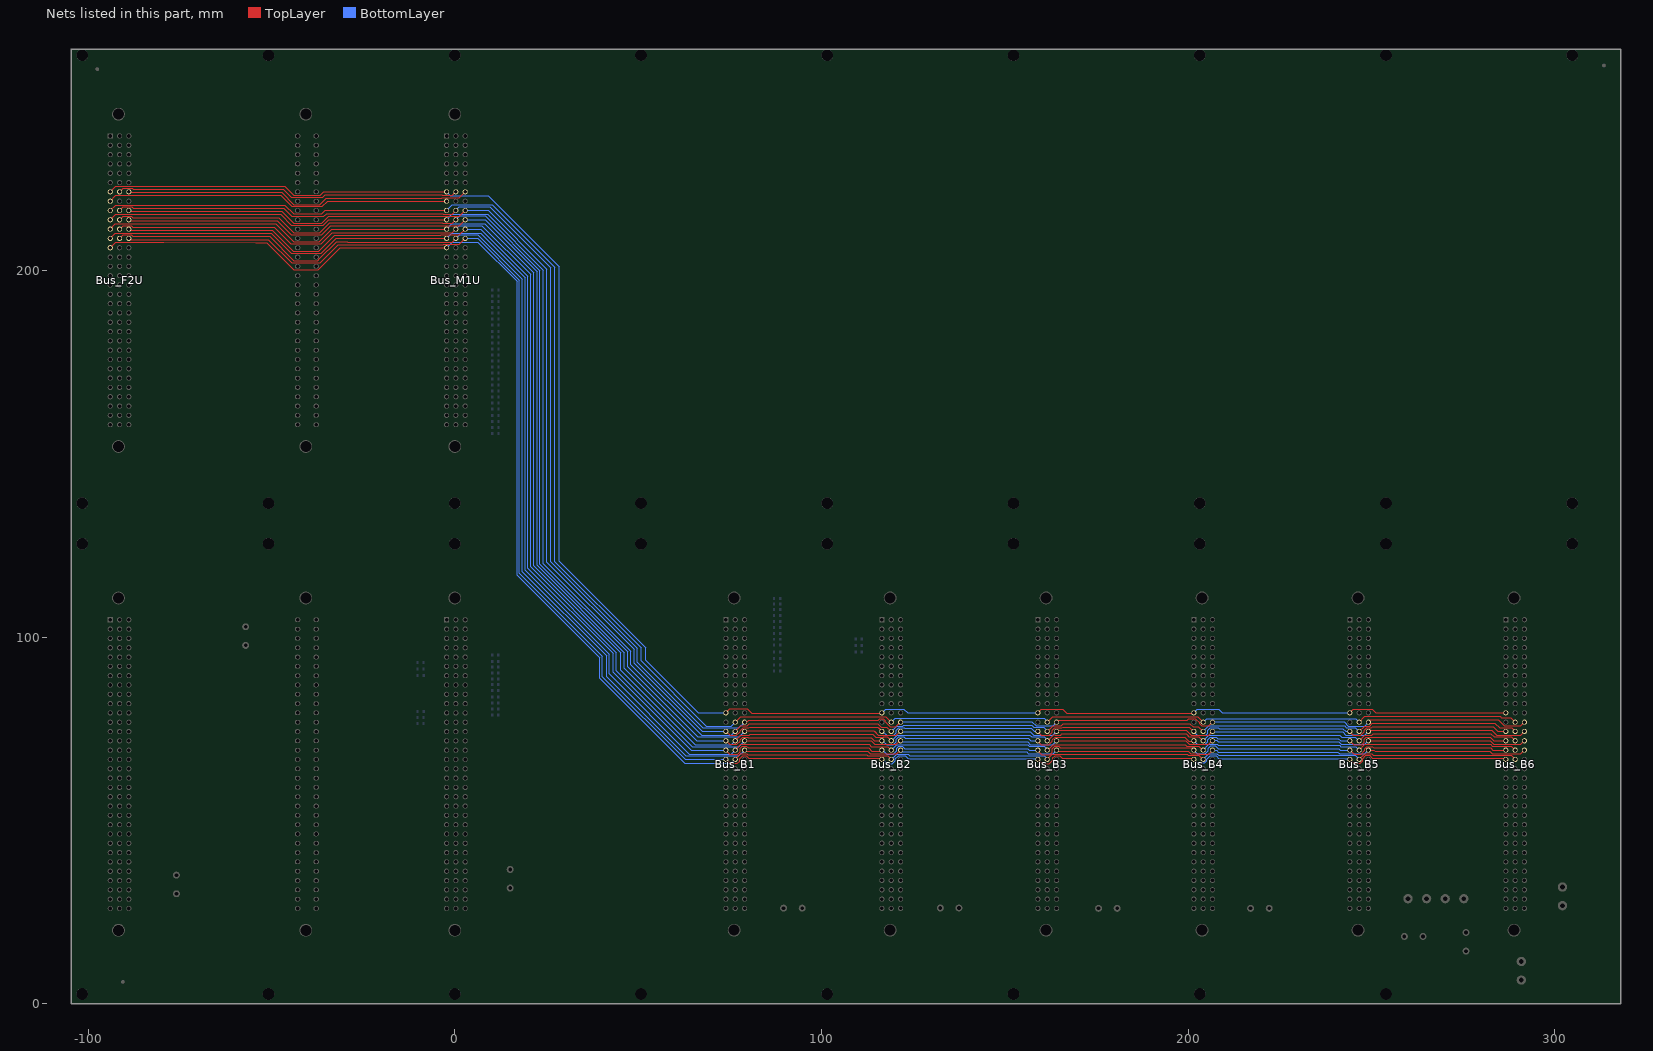
[diagram p0: the nets of this part, all layers, seen from the top]
# Altium PCB MISC67337.PcbDoc (part 5 of 7)
Units mm, origin at the board's own origin, x right, y up, seen from the top; angles counter-clockwise.
Board outline 422.71 x 260.35 mm, 4 copper layers (TopLayer, InternalPlane1, InternalPlane2, BottomLayer); 82 components, 143 nets, 1295 pads, 42 vias.

## Via types
v1: diameter 0.61, hole 0.305, TopLayer to BottomLayer, 42 vias

## Nets (pads, with @x,y where several pads share a name; then routed paths per layer and width w, separated by ;. In a path a pad name is that pad's centre, name@x,y a point inside that pad or via, vN(x,y) a via of type N, cw(c..) or ccw(c..) an arc to the next point about the centre after c; other vN are vias at no path point) (continued)
B_DSP2_XA12: Bus_B1.A11 Bus_B2.A11 Bus_B3.A11 Bus_B4.A11 Bus_B5.A11 Bus_B6.A11 Bus_F2U.A7 Bus_M1U.A7 | length 496.5
  TopLayer w0.254: Bus_F2U.A7@-93.97,221.413 -92.407,222.976 ; -92.407,222.965 -46.384,222.965 -43.891,220.472 -36.703,220.472 -35.762,221.413 -34.544,221.413 ; -35.285,221.413 -34.544,221.413 ; Bus_M1U.A7@-2.373,221.28 Bus_M1U.A7@-2.24,221.413 ; Bus_M1U.A7@-2.373,221.413 -34.544,221.413 ; Bus_B1.A11@73.96,79.44 74.938,80.418 79.754,80.418 80.964,79.208 81.661,79.208 ; 81.117,79.208 81.661,79.208 ; Bus_B2.A11@116.316,79.208 81.661,79.208 ; Bus_B2.A11@116.316,79.502 Bus_B2.A11@116.505,79.313 ; Bus_B3.A11@159.05,79.313 160.028,80.291 165.835,80.291 166.879,79.247 Bus_B4.A11@201.406,79.247 ; Bus_B4.A11@201.406,79.375 Bus_B4.A11@201.595,79.186 ; Bus_B5.A11@244.14,79.313 245.118,80.291 250.214,80.291 251.193,79.312 Bus_B6.A11@286.685,79.312
  BottomLayer w0.254: Bus_M1U.A7@-2.24,221.413 -1.172,220.345 9.144,220.345 28.448,201.041 28.448,120.65 52.07,97.028 52.07,93.599 66.356,79.313 Bus_B1.A11@73.955,79.313 ; Bus_B2.A11@116.632,79.375 117.61,80.353 122.453,80.353 123.493,79.313 Bus_B3.A11@159.05,79.313 ; Bus_B3.A11@159.144,79.408 Bus_B3.A11@159.177,79.375 ; Bus_B4.A11@201.595,79.313 202.548,80.266 203.706,80.266 ; 203.73,80.291 207.188,80.291 ; 207.467,80.291 207.188,80.291 ; Bus_B5.A11@244.14,79.313 209.383,79.313 208.405,80.291 207.188,80.291
B_DSP2_XA13: Bus_F2U.B7 Bus_M1U.B7 | length 98.4
  TopLayer w0.254: Bus_F2U.B7@-91.43,221.413 -90.452,222.391 -88.001,222.391 -87.732,222.122 -49.581,222.122 ; -47.255,222.122 -49.581,222.122 ; -35.012,220.567 -32.817,220.567 ; Bus_M1U.B7@0.3,221.413 -0.678,220.436 -3.469,220.436 -3.6,220.567 -32.817,220.567 ; -49.581,222.122 -46.76,222.122 -44.602,219.964 -35.992,219.964 -35.389,220.567 -32.817,220.567
B_DSP2_XA14: Bus_F2U.C7 Bus_M1U.C7 | length 94.5
  TopLayer w0.254: Bus_F2U.C7@-88.89,221.279 -47.187,221.279 -43.867,217.959 -36.803,217.959 -35.042,219.72 -3.521,219.72 -3.389,219.851 1.278,219.851 Bus_M1U.C7@2.84,221.413
B_DSP2_XA15: Bus_F2U.A8 Bus_M1U.A8 | length 94.2
  TopLayer w0.254: Bus_F2U.A8@-93.97,218.873 -92.407,220.436 -47.487,220.436 -44.475,217.424 -36.119,217.424 -34.669,218.873 Bus_M1U.A8@-2.24,218.873
B_DSP2_XD0: Bus_B1.B12 Bus_B2.B12 Bus_B3.B12 Bus_B4.B12 Bus_B5.B12 Bus_B6.B12 Bus_F2U.A9 Bus_M1U.A9 | length 503.7
  TopLayer w0.254: Bus_F2U.A9@-93.97,216.333 -92.498,217.805 -46.355,217.805 -43.942,215.392 -36.271,215.392 -35.33,216.333 Bus_M1U.A9@-2.24,216.333 ; Bus_B1.B12@76.495,76.773 77.984,78.262 117.556,78.262 Bus_B2.B12@119.045,76.773 ; 162.974,78.157 Bus_B3.B12@161.59,76.773 163.115,78.298 202.61,78.298 Bus_B4.B12@204.135,76.773 202.751,78.157 ; Bus_B5.B12@246.68,76.773 248.242,78.335 249.625,78.335 249.65,78.36 285.14,78.36 285.471,78.029 287.969,78.029 Bus_B6.B12@289.225,76.773
  BottomLayer w0.254: Bus_M1U.A9@-2.24,216.333 -0.678,217.896 10.247,217.896 27.305,200.838 27.305,120.523 50.8,97.028 50.8,93.472 68.58,75.692 75.414,75.692 Bus_B1.B12@76.495,76.773 ; Bus_B2.B12@119.172,76.835 120.15,77.813 160.739,77.813 Bus_B3.B12@161.717,76.835 ; Bus_B4.B12@204.135,76.773 205.113,77.751 245.702,77.751 Bus_B5.B12@246.68,76.773
B_DSP2_XD1: Bus_B1.C12 Bus_B2.C12 Bus_B3.C12 Bus_B4.C12 Bus_B5.C12 Bus_B6.C12 Bus_F2U.B9 Bus_M1U.B9 | length 504.6
  TopLayer w0.254: Bus_F2U.B9@-91.43,216.333 -90.452,217.311 -88.093,217.311 -87.732,216.95 -46.592,216.95 -44.399,214.757 -35.712,214.757 -34.983,215.487 -3.219,215.487 -3.088,215.356 -0.678,215.356 Bus_M1U.B9@0.3,216.333 ; Bus_B1.C12@79.035,76.773 79.67,76.773 80.213,77.316 112.547,77.316 ; 114.111,77.316 112.547,77.316 ; Bus_B2.C12@121.585,76.9 120.25,75.565 118.745,75.565 117.483,76.827 117.483,77.178 116.91,77.751 115.978,77.751 115.543,77.316 112.547,77.316 ; Bus_B3.C12@164.13,76.808 164.165,76.808 164.707,77.35 197.587,77.35 ; 199.201,77.35 197.587,77.35 ; Bus_B4.C12@206.675,76.773 205.697,75.795 203.73,75.795 203.157,76.368 203.157,76.594 202,77.751 200.179,77.751 199.778,77.35 197.587,77.35 ; Bus_B5.C12@249.22,76.773 249.854,77.407 284.644,77.407 286.256,75.795 290.787,75.795 Bus_B6.C12@291.765,76.773
  BottomLayer w0.254: Bus_M1U.B9@0.3,216.333 1.278,217.311 9.536,217.311 26.162,200.685 26.162,120.523 49.784,96.901 49.784,93.091 67.664,75.211 77.473,75.211 Bus_B1.C12@79.035,76.773 ; Bus_B2.C12@121.712,76.897 157.418,76.897 158.536,75.779 163.201,75.779 Bus_B3.C12@164.257,76.835 ; Bus_B4.C12@206.675,76.839 242.591,76.839 243.713,75.717 248.164,75.717 Bus_B5.C12@249.22,76.773
B_DSP2_XD2: Bus_B1.A13 Bus_B2.A13 Bus_B3.A13 Bus_B4.A13 Bus_B5.A13 Bus_B6.A13 Bus_F2U.C9 Bus_M1U.C9 | length 502.2
  TopLayer w0.254: Bus_F2U.C9@-88.89,216.095 -48.514,216.095 ; -47.804,216.095 -48.514,216.095 ; Bus_M1U.C9@2.84,216.333 1.278,214.771 -34.403,214.771 -36.295,212.879 -43.921,212.879 -47.137,216.095 -48.514,216.095 ; Bus_B1.A13@73.96,74.36 75.168,73.152 76.835,73.152 77.851,74.168 77.851,74.432 78.63,75.211 80.188,75.211 80.401,75.424 115.314,75.424 Bus_B2.A13@116.505,74.233 ; 115.654,75.211 Bus_B2.A13@116.505,74.36 ; Bus_B3.A13@159.05,74.233 160.028,73.255 162.155,73.255 162.941,74.041 162.941,74.549 163.603,75.211 165.583,75.211 165.825,75.453 200.375,75.453 Bus_B4.A13@201.595,74.233 200.517,75.311 ; Bus_B5.A13@244.14,74.233 245.118,73.255 247.118,73.255 248.031,74.168 248.031,74.549 248.693,75.211 250.038,75.211 250.329,75.502 283.273,75.502 284.542,74.233 Bus_B6.A13@286.685,74.233
  BottomLayer w0.254: Bus_M1U.C9@2.84,216.333 9.168,216.333 25.146,200.355 25.146,120.396 48.895,96.647 48.895,92.837 67.499,74.233 Bus_B1.A13@73.955,74.233 ; Bus_B2.A13@116.632,74.295 117.775,73.152 119.699,73.152 120.396,73.849 120.396,74.611 121.071,75.286 122.407,75.286 122.582,75.286 122.803,75.065 155.956,75.065 ; 156.972,75.065 155.956,75.065 ; Bus_B3.A13@159.177,74.295 158.05,74.295 157.28,75.065 155.956,75.065 ; Bus_B4.A13@201.595,74.233 202.573,73.255 204.827,73.255 205.359,73.787 205.359,74.549 206.032,75.222 ; 206.121,75.222 206.032,75.222 ; 241.935,75.015 241.198,75.015 ; Bus_B5.A13@244.14,74.233 243.013,74.233 242.231,75.015 241.198,75.015 ; 206.032,75.222 206.07,75.26 208.289,75.26 208.534,75.015 241.198,75.015
B_DSP2_XD3: Bus_B1.B13 Bus_B2.B13 Bus_B3.B13 Bus_B4.B13 Bus_B5.B13 Bus_B6.B13 Bus_F2U.A10 Bus_M1U.A10 | length 506.3
  TopLayer w0.254: Bus_F2U.A10@-93.97,213.793 -92.523,215.24 -47.498,215.24 -44.602,212.344 -35.814,212.344 -34.365,213.793 Bus_M1U.A10@-2.315,213.793 ; Bus_M1U.A10@-2.315,213.868 Bus_M1U.A10@-2.24,213.793 ; Bus_B1.B13@76.495,74.233 78.057,75.795 79.807,75.795 80.382,76.37 115.4,76.37 116.332,75.438 ; Bus_B1.B13@76.5,74.233 77.46,75.194 ; 116.068,75.702 116.332,75.438 ; Bus_B2.B13@119.045,74.233 117.84,75.438 116.332,75.438 ; Bus_B3.B13@161.653,74.17 163.302,75.818 ; 163.424,75.818 163.447,75.795 165.408,75.795 166.014,76.402 200.509,76.402 201.379,75.532 202.836,75.532 Bus_B4.B13@204.135,74.233 ; Bus_B4.B13@204.071,74.17 Bus_B4.B13@204.135,74.106 ; Bus_B5.B13@246.68,74.233 248.139,75.692 249.522,75.692 250.285,76.455 252.603,76.455 ; 250.698,76.455 252.603,76.455 ; Bus_B6.B13@289.225,74.233 288.247,75.211 284.961,75.211 283.717,76.455 252.603,76.455
  BottomLayer w0.254: Bus_M1U.A10@-2.24,213.793 -0.768,215.265 8.966,215.265 24.13,200.101 24.13,120.015 48.006,96.139 48.006,92.456 67.31,73.152 75.414,73.152 Bus_B1.B13@76.495,74.233 ; Bus_B2.B13@119.172,74.295 120.569,75.692 122.239,75.692 122.528,75.981 157.318,75.981 157.926,75.373 160.639,75.373 Bus_B3.B13@161.717,74.295 ; Bus_B4.B13@204.135,74.233 205.697,75.795 242.721,75.795 243.205,75.311 245.602,75.311 Bus_B5.B13@246.68,74.233
B_DSP2_XD4: Bus_B1.C13 Bus_B2.C13 Bus_B3.C13 Bus_B4.C13 Bus_B5.C13 Bus_B6.C13 Bus_F2U.B10 Bus_M1U.B10 | length 502.2
  TopLayer w0.254: Bus_F2U.B10@-91.43,213.793 -90.441,214.782 -88.18,214.782 -87.782,214.384 ; -87.808,214.384 -87.782,214.384 ; Bus_M1U.B10@0.3,213.793 -0.678,212.816 -3.291,212.816 -3.422,212.947 -34.144,212.947 -36.779,210.312 -43.891,210.312 -47.964,214.384 -87.782,214.384 ; Bus_B1.C13@79.04,74.478 114.244,74.478 115.456,73.266 ; 114.489,74.233 115.456,73.266 ; Bus_B2.C13@121.585,74.36 120.377,73.152 115.57,73.152 115.456,73.266 ; Bus_B3.C13@164.13,74.505 199.563,74.505 200.812,73.255 205.697,73.255 Bus_B4.C13@206.675,74.233 ; Bus_B5.C13@249.22,74.233 Bus_B5.C13@249.282,74.295 ; Bus_B5.C13@249.282,74.55 282.904,74.55 284.199,73.255 290.787,73.255 Bus_B6.C13@291.765,74.233
  BottomLayer w0.254: Bus_M1U.B10@0.3,213.793 1.365,214.859 8.306,214.859 23.241,199.923 23.241,119.888 47.117,96.012 47.117,91.948 66.319,72.746 77.548,72.746 Bus_B1.C13@79.035,74.233 ; Bus_B2.C13@121.712,74.149 156.926,74.149 157.923,73.152 163.114,73.152 Bus_B3.C13@164.257,74.295 ; Bus_B4.C13@206.675,74.103 209.499,74.103 242.203,74.103 243.051,73.255 244.832,73.255 244.856,73.279 246.251,73.279 246.275,73.255 248.242,73.255 Bus_B5.C13@249.22,74.233
B_DSP2_XD5: Bus_B1.A14 Bus_B2.A14 Bus_B3.A14 Bus_B4.A14 Bus_B5.A14 Bus_B6.A14 Bus_F2U.C10 Bus_M1U.C10 | length 501.1
  TopLayer w0.254: Bus_F2U.C10@-88.89,213.529 -50.267,213.529 ; -49.074,213.529 -50.267,213.529 ; Bus_M1U.C10@2.84,213.793 1.278,212.231 -33.768,212.231 -36.322,209.677 -44.552,209.677 -48.404,213.529 -50.267,213.529 ; Bus_B1.A14@73.96,71.693 74.938,70.715 76.938,70.715 77.851,71.628 77.851,72.009 78.513,72.671 79.907,72.671 79.991,72.587 113.545,72.587 114.402,71.73 116.468,71.73 Bus_B2.A14@116.505,71.693 ; Bus_B3.A14@159.05,71.566 160.028,70.588 162.028,70.588 162.941,71.501 162.941,71.882 163.152,72.093 163.152,72.098 163.725,72.671 199.123,72.671 200.228,71.566 201.468,71.566 Bus_B4.A14@201.595,71.693 ; Bus_B5.A14@244.14,71.693 245.221,70.612 247.396,70.612 248.031,71.247 248.031,72.136 248.566,72.671 282.421,72.671 283.399,71.693 Bus_B6.A14@286.685,71.693
  BottomLayer w0.254: Bus_M1U.C10@2.84,213.793 8.304,213.793 22.479,199.619 22.479,119.507 46.228,95.758 46.228,91.44 65.975,71.693 Bus_B1.A14@73.955,71.693 ; Bus_B2.A14@116.632,71.755 117.775,70.612 119.572,70.612 120.396,71.436 120.396,72.071 121.058,72.733 122.492,72.733 122.907,72.317 154.686,72.317 ; 155.705,72.317 154.686,72.317 ; Bus_B3.A14@159.177,71.755 157.037,71.755 156.475,72.317 154.686,72.317 ; Bus_B4.A14@201.595,71.693 202.573,70.715 204.7,70.715 205.359,71.374 205.359,72.009 206.021,72.671 207.72,72.671 208.111,72.28 239.116,72.28 ; 240.668,72.28 239.116,72.28 ; Bus_B5.A14@244.14,71.693 241.616,71.693 241.029,72.28 239.116,72.28
B_DSP2_XD6: Bus_B1.B14 Bus_B2.B14 Bus_B3.B14 Bus_B4.B14 Bus_B5.B14 Bus_B6.B14 Bus_F2U.A11 Bus_M1U.A11 | length 509.3
  TopLayer w0.254: Bus_F2U.A11@-93.97,211.253 -92.549,212.674 -50.597,212.674 ; -50.419,212.674 -50.597,212.674 ; Bus_M1U.A11@-2.24,211.253 -33.526,211.253 -36.981,207.799 -37.616,207.799 -37.643,207.772 -43.942,207.772 -48.844,212.674 -50.597,212.674 ; Bus_B1.B14@76.5,71.693 78.035,73.228 80.315,73.228 80.619,73.532 114.072,73.532 114.884,72.72 116.942,72.72 116.967,72.746 ; 116.942,72.746 116.967,72.746 ; Bus_B2.B14@119.045,71.693 117.992,72.746 116.967,72.746 ; Bus_B3.B14@161.59,71.566 162.919,72.895 ; 163.201,73.177 162.919,72.895 ; 199.873,73.177 200.19,72.86 ; Bus_B4.B14@204.135,71.566 202.93,72.771 200.279,72.771 200.19,72.86 ; Bus_B5.B14@246.68,71.693 248.139,73.152 250.063,73.152 250.508,73.597 282.638,73.597 283.464,72.771 288.147,72.771 Bus_B6.B14@289.225,71.693 ; 162.919,72.895 163.354,73.33 163.65,73.33 163.725,73.255 165.229,73.255 165.53,73.557 199.493,73.557 200.19,72.86
  BottomLayer w0.254: Bus_M1U.A11@-2.24,211.253 -0.768,212.725 8.179,212.725 21.59,199.314 21.59,119.38 45.212,95.758 45.212,90.932 65.532,70.612 75.414,70.612 Bus_B1.B14@76.495,71.693 ; Bus_B2.B14@119.172,71.755 120.65,73.233 124.282,73.233 ; 123.063,73.233 124.282,73.233 ; 156.337,73.233 155.143,73.233 ; Bus_B3.B14@161.717,71.755 160.726,72.746 157.313,72.746 156.826,73.233 155.143,73.233 ; Bus_B4.B14@204.135,71.693 205.634,73.192 209.728,73.192 ; 208.026,73.192 209.728,73.192 ; Bus_B5.B14@246.68,71.693 245.653,72.72 241.884,72.72 241.413,73.192 239.141,73.192 209.728,73.192 ; 124.282,73.233 155.143,73.233
B_DSP2_XD7: Bus_B1.C14 Bus_B2.C14 Bus_B3.C14 Bus_B4.C14 Bus_B5.C14 Bus_B6.C14 Bus_F2U.B11 Bus_M1U.B11 | length 507.6
  TopLayer w0.254: Bus_F2U.B11@-91.43,211.253 -90.452,212.231 -88.296,212.231 -87.884,211.819 -51.638,211.819 ; -50.038,211.819 -51.638,211.819 ; Bus_M1U.B11@0.3,211.253 -0.678,210.276 -33.361,210.276 -36.373,207.264 -44.729,207.264 -49.284,211.819 -51.638,211.819 ; Bus_B1.C14@79.04,71.693 Bus_B1.C14@79.102,71.755 ; Bus_B1.C14@79.102,71.641 113.603,71.641 114.529,70.715 ; 114.503,70.715 114.529,70.715 ; Bus_B2.C14@121.585,71.82 120.48,70.715 114.529,70.715 ; Bus_B3.C14@164.13,71.566 Bus_B3.C14@164.192,71.628 ; Bus_B3.C14@164.192,71.66 199.333,71.66 200.277,70.715 205.697,70.715 Bus_B4.C14@206.675,71.693 ; Bus_B5.C14@249.22,71.693 282.45,71.693 283.428,70.715 290.787,70.715 Bus_B6.C14@291.765,71.693
  BottomLayer w0.254: Bus_M1U.B11@0.3,211.253 1.278,212.231 3.245,212.231 3.259,212.217 7.366,212.217 20.701,198.882 20.701,119.126 44.069,95.758 44.069,90.805 64.743,70.131 77.473,70.131 Bus_B1.C14@79.035,71.693 ; Bus_B2.C14@121.585,71.693 121.952,72.06 121.952,71.401 154.28,71.401 ; 155.194,71.401 154.28,71.401 ; Bus_B3.C14@164.257,71.755 163.114,70.612 157.034,70.612 156.245,71.401 154.28,71.401 ; Bus_B4.C14@206.675,71.693 206.788,71.806 207.772,71.806 208.21,71.368 210.896,71.368 ; 208.661,71.368 210.896,71.368 ; 240.157,71.368 239.268,71.368 ; Bus_B5.C14@249.22,71.693 248.242,70.715 241.832,70.715 241.179,71.368 239.268,71.368 ; 210.896,71.368 239.268,71.368
B_DSP2_XD8: Bus_B1.A15 Bus_B2.A15 Bus_B3.A15 Bus_B4.A15 Bus_B5.A15 Bus_B6.A15 Bus_F2U.C11 Bus_M1U.C11 | length 513.3
  TopLayer w0.254: Bus_F2U.C11@-88.89,210.964 -51.283,210.964 ; -50.217,210.964 -51.283,210.964 ; -30.899,209.56 -25.527,209.56 ; Bus_M1U.C11@2.84,211.247 Bus_M1U.C11@2.84,211.253 1.278,209.691 -3.653,209.691 -3.785,209.56 -25.527,209.56 ; Bus_B1.A15@73.96,69.153 75.041,68.072 77.216,68.072 77.851,68.707 77.851,69.596 78.461,70.206 79.527,70.206 79.984,69.749 82.169,69.749 ; 80.772,69.749 82.169,69.749 ; 111.887,69.749 111.1,69.749 ; Bus_B2.A15@116.505,69.153 116.237,68.885 113.767,68.885 112.903,69.749 111.1,69.749 ; Bus_B3.A15@159.05,69.026 160.131,67.945 162.306,67.945 162.941,68.58 162.941,69.469 163.703,70.231 164.719,70.231 165.187,69.763 167.411,69.763 ; 165.862,69.763 167.411,69.763 ; 196.977,69.763 196.825,69.763 ; Bus_B4.A15@201.595,69.153 200.985,69.763 196.825,69.763 ; Bus_B5.A15@244.14,69.153 244.283,69.153 245.364,68.072 247.269,68.072 248.242,69.045 248.242,69.558 248.815,70.131 250.304,70.131 250.647,69.788 280.568,69.788 ; 281.913,69.788 280.568,69.788 ; Bus_B6.A15@286.685,69.153 283.145,69.153 282.51,69.788 280.568,69.788 ; -51.283,210.964 -49.75,210.964 -44.018,205.232 -37.059,205.232 -32.731,209.56 -25.527,209.56 ; 82.169,69.749 111.1,69.749 ; 167.411,69.763 196.825,69.763
  BottomLayer w0.254: Bus_M1U.C11@2.84,211.253 7.085,211.253 19.939,198.399 19.939,118.745 43.18,95.504 43.18,90.424 64.451,69.153 Bus_B1.A15@73.955,69.153 ; Bus_B2.A15@116.632,69.215 117.775,68.072 119.572,68.072 120.523,69.023 120.523,69.658 121.071,70.206 122.072,70.206 122.709,69.569 124.409,69.569 ; 124.206,69.569 124.409,69.569 ; 154.686,69.569 154.102,69.569 ; Bus_B3.A15@159.05,69.153 156.653,69.153 156.237,69.569 154.102,69.569 ; Bus_B3.A15@159.05,69.215 Bus_B3.A15@159.177,69.215 ; Bus_B4.A15@201.595,69.153 202.573,68.175 204.7,68.175 205.486,68.961 205.486,69.596 206.199,70.309 207.415,70.309 208.179,69.544 209.575,69.544 ; 209.169,69.544 209.575,69.544 ; 239.649,69.544 239.293,69.544 ; Bus_B5.A15@244.14,69.153 241.489,69.153 241.098,69.544 239.293,69.544 ; 124.409,69.569 154.102,69.569 ; 209.575,69.544 239.293,69.544
B_DSP2_XD9: Bus_B1.B15 Bus_B2.B15 Bus_B3.B15 Bus_B4.B15 Bus_B5.B15 Bus_B6.B15 Bus_F2U.A12 Bus_M1U.A12 | length 513.4
  TopLayer w0.254: Bus_F2U.A12@-93.97,208.713 -92.574,210.109 -50.038,210.109 -44.653,204.724 -36.373,204.724 -32.383,208.713 Bus_M1U.A12@-2.24,208.713 ; Bus_B1.B15@76.5,69.153 78.042,70.695 84.709,70.695 ; 80.391,70.695 84.709,70.695 ; 112.395,70.695 111.277,70.695 ; Bus_B2.B15@119.045,69.153 118.067,70.131 116.1,70.131 116.098,70.129 113.614,70.129 113.049,70.695 111.277,70.695 ; Bus_B3.B15@161.59,69.026 163.201,70.637 199.238,70.637 199.644,70.231 202.93,70.231 Bus_B4.B15@204.135,69.026 ; Bus_B5.B15@246.68,69.153 248.267,70.74 248.79,70.74 248.815,70.715 253.569,70.715 253.594,70.74 ; 250.444,70.74 253.594,70.74 ; Bus_B6.B15@289.225,69.153 288.147,70.231 283.032,70.231 282.523,70.74 253.594,70.74 ; 84.709,70.695 111.277,70.695
  BottomLayer w0.254: Bus_M1U.A12@-2.24,208.713 -0.768,210.185 7.036,210.185 19.177,198.044 19.177,118.237 42.164,95.25 42.164,89.916 64.008,68.072 75.414,68.072 Bus_B1.B15@76.495,69.153 ; Bus_B2.B15@119.172,69.215 120.569,70.612 156.275,70.612 156.694,70.193 160.739,70.193 Bus_B3.B15@161.717,69.215 ; Bus_B4.B15@204.135,69.153 205.697,70.715 207.948,70.715 208.207,70.456 239.243,70.456 ; 240.16,70.456 239.243,70.456 ; Bus_B5.B15@246.68,69.153 245.702,70.131 243.735,70.131 243.708,70.104 241.684,70.104 241.332,70.456 239.243,70.456
B_DSP2_XD10: Bus_B1.C15 Bus_B2.C15 Bus_B3.C15 Bus_B4.C15 Bus_B5.C15 Bus_B6.C15 Bus_F2U.B12 Bus_M1U.B12 | length 508.7
  TopLayer w0.254: Bus_F2U.B12@-91.43,208.713 -90.452,209.691 -88.271,209.691 -87.833,209.254 -50.529,209.254 -43.967,202.692 -37.321,202.692 -36.759,203.255 -36.759,203.271 -32.163,207.867 -29.362,207.867 ; -30.389,207.867 -29.362,207.867 ; Bus_M1U.B12@0.3,208.713 -0.678,207.736 -29.231,207.736 -29.362,207.867 ; Bus_B1.C15@79.04,68.803 111.912,68.803 ; 112.27,68.803 111.912,68.803 ; Bus_B2.C15@121.585,69.153 120.529,68.097 113.386,68.097 112.68,68.803 111.912,68.803 ; Bus_B3.C15@164.13,68.815 197.256,68.815 ; 197.36,68.815 197.256,68.815 ; Bus_B4.C15@206.675,69.026 205.721,68.072 203.124,68.072 203.098,68.097 200.736,68.097 200.019,68.815 197.256,68.815 ; Bus_B5.C15@249.22,69.153 250.685,69.153 251.003,68.835 277.343,68.835 ; 280.605,68.835 277.343,68.835 ; Bus_B6.C15@291.765,69.153 290.787,68.175 282.956,68.175 282.296,68.835 277.343,68.835
  BottomLayer w0.254: Bus_M1U.B12@0.3,208.713 1.365,209.779 6.248,209.779 18.415,197.612 18.415,117.856 41.402,94.869 41.402,89.154 62.965,67.591 77.473,67.591 Bus_B1.C15@79.035,69.153 ; Bus_B2.C15@121.712,68.653 154.762,68.653 ; 155.383,68.653 154.762,68.653 ; Bus_B3.C15@164.257,69.215 163.216,68.174 156.424,68.174 155.945,68.653 154.762,68.653 ; Bus_B4.C15@206.675,69.153 207.783,69.153 208.304,68.632 239.827,68.632 ; 240.346,68.632 239.827,68.632 ; Bus_B5.C15@249.22,69.153 248.242,68.175 241.324,68.175 240.867,68.632 239.827,68.632
B_DSP2_XD11: Bus_B1.A16 Bus_B2.A16 Bus_B3.A16 Bus_B4.A16 Bus_B5.A16 Bus_B6.A16 Bus_F2U.C12 Bus_M1U.C12 | length 508.2
  TopLayer w0.254: Bus_F2U.C12@-88.89,208.399 -52.045,208.399 ; -51.611,208.399 -52.045,208.399 ; -29.972,207.02 -29.007,207.02 ; 1.391,207.264 Bus_M1U.C12@2.84,208.713 1.278,207.151 -3.044,207.151 -3.175,207.02 -29.007,207.02 ; Bus_B1.A16@73.96,66.613 74.103,66.613 75.184,65.532 77.089,65.532 77.724,66.167 77.724,66.807 78.508,67.591 79.44,67.591 80.12,66.911 111.379,66.911 ; 111.606,66.911 111.379,66.911 ; Bus_B2.A16@116.505,66.613 116.207,66.911 111.379,66.911 ; Bus_B3.A16@159.05,66.486 159.193,66.486 160.274,65.405 162.179,65.405 163.152,66.378 163.152,67.018 163.725,67.591 163.882,67.591 163.906,67.615 164.987,67.615 165.684,66.918 195.809,66.918 ; 196.696,66.918 195.809,66.918 ; Bus_B4.A16@201.468,66.486 Bus_B4.A16@201.595,66.613 201.29,66.918 195.809,66.918 ; Bus_B5.A16@244.14,66.613 245.221,65.532 246.982,65.532 247.658,66.208 247.658,66.81 248.539,67.691 249.53,67.691 250.29,66.93 251.409,66.93 ; 250.825,66.93 251.409,66.93 ; 279.273,66.93 279.095,66.93 ; Bus_B6.A16@286.685,66.613 286.65,66.613 286.334,66.929 279.097,66.929 279.095,66.93 ; -52.045,208.399 -50.868,208.399 -44.526,202.057 -36.703,202.057 -31.74,207.02 -29.007,207.02 ; 251.409,66.93 279.095,66.93
  BottomLayer w0.254: Bus_M1U.C12@2.84,208.713 6.272,208.713 17.653,197.333 17.653,117.348 40.259,94.742 40.259,89.154 62.8,66.613 Bus_B1.A16@73.955,66.613 ; Bus_B2.A16@116.632,66.675 117.902,65.405 119.285,65.405 120.15,66.27 120.15,66.745 121.058,67.653 122.898,67.653 123.73,66.821 154.127,66.821 ; 155.067,66.821 154.127,66.821 ; Bus_B3.A16@159.05,66.613 Bus_B3.A16@158.988,66.675 ; Bus_B3.A16@159.177,66.675 Bus_B3.A16@158.988,66.675 ; Bus_B4.A16@201.595,66.613 202.549,65.659 203.706,65.659 203.73,65.635 204.54,65.635 205.113,66.208 205.113,66.683 206.021,67.591 207.643,67.591 208.426,66.809 238.709,66.809 ; 240.03,66.809 238.709,66.809 ; Bus_B5.A16@244.14,66.613 243.944,66.809 238.709,66.809 ; 154.127,66.821 158.842,66.821 Bus_B3.A16@158.988,66.675
B_DSP2_XD12: Bus_B1.B16 Bus_B2.B16 Bus_B3.B16 Bus_B4.B16 Bus_B5.B16 Bus_B6.B16 Bus_F2U.A13 Bus_M1U.A13 | length 513.7
  TopLayer w0.254: Bus_F2U.A13@-93.865,206.173 Bus_F2U.A13@-93.97,206.173 -92.52,207.623 -79.375,207.623 -54.28,207.55 ; -52.161,207.543 -54.28,207.55 ; Bus_M1U.A13@-2.24,206.173 -31.19,206.173 -37.211,200.152 -43.917,200.152 -51.314,207.55 -54.28,207.55 ; Bus_B1.B16@76.5,66.613 78.011,68.124 79.705,68.124 79.973,67.857 112.395,67.857 112.662,67.589 116.098,67.589 116.1,67.591 118.067,67.591 Bus_B2.B16@119.045,66.613 ; Bus_B3.B16@161.59,66.486 Bus_B3.B16@161.653,66.55 ; Bus_B3.B16@161.59,66.613 163.024,68.047 199.746,68.047 200.101,67.691 202.93,67.691 Bus_B4.B16@204.135,66.486 ; Bus_B5.B16@246.68,66.613 248.164,68.097 250.088,68.097 250.495,67.691 285.039,67.691 ; 280.67,67.691 285.039,67.691 ; Bus_B6.B16@289.225,66.613 288.147,67.691 285.039,67.691
  BottomLayer w0.254: Bus_M1U.A13@-2.24,206.173 -0.678,207.736 6.285,207.736 17.018,197.002 17.018,116.84 39.497,94.361 39.497,88.773 62.738,65.532 75.414,65.532 Bus_B1.B16@76.495,66.613 ; Bus_B2.B16@119.172,66.675 120.569,68.072 122.149,68.072 123.673,68.072 124.13,67.615 160.833,67.615 161.835,66.613 Bus_B3.B16@161.59,66.613 ; Bus_B3.B16@161.684,66.708 Bus_B3.B16@161.717,66.675 ; Bus_B4.B16@204.135,66.613 205.697,68.175 207.876,68.175 208.331,67.72 239.344,67.72 ; 240.157,67.72 239.344,67.72 ; Bus_B5.B16@246.68,66.613 245.573,67.72 239.344,67.72